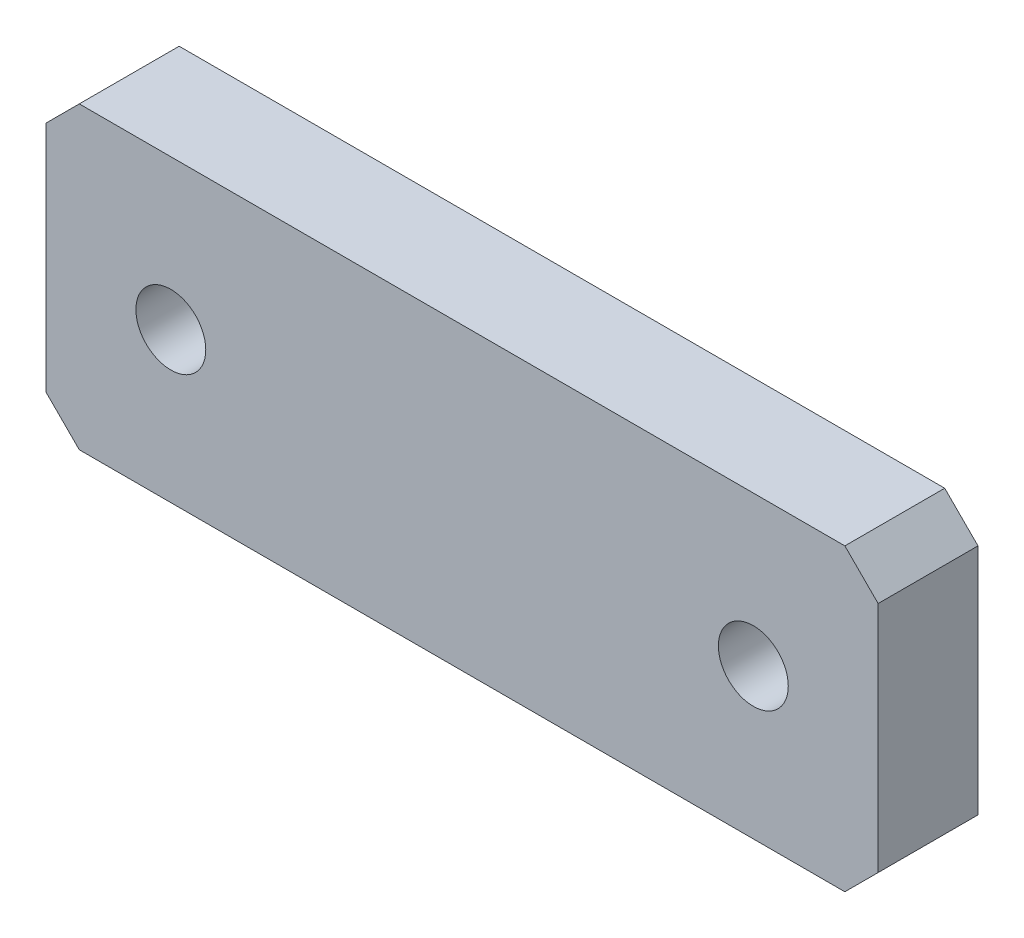
from build123d import *

# Parameters (mm, degrees)
SKETCH1_W           = 50
SKETCH1_H           = 18
BOSS_EXTRUDE1_DEPTH = 3
M5_TAPPED_HOLE1_D   = 4.2
CHAMFER1_SIZE       = 2


with BuildPart() as part:
    # Sketch1 → Boss-Extrude1 (new, symmetric)
    with BuildSketch(Plane.XY):
        Rectangle(SKETCH1_W, SKETCH1_H)
    extrude(amount=BOSS_EXTRUDE1_DEPTH, both=True)

    # M5 Tapped Hole1 (through all)
    with Locations(Plane.XY.offset(3)):
        with Locations((-17.5, 0), (17.5, 0)):
            Hole(M5_TAPPED_HOLE1_D / 2)

    # Chamfer1
    chamfer1_edges = [part.edges().sort_by_distance(p)[0] for p in [
        (-25, 9, 0),
        (25, 9, 0),
        (25, -9, 0),
        (-25, -9, 0),
    ]]
    chamfer(chamfer1_edges, length=CHAMFER1_SIZE)


solid = part.part
